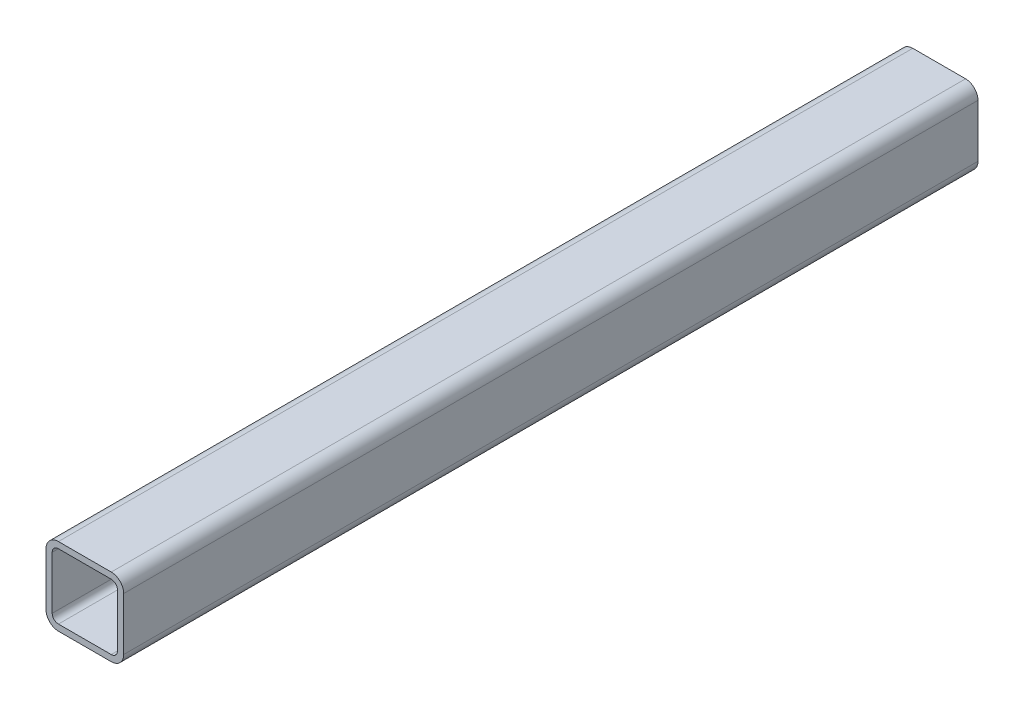
from build123d import *

# Parameters (mm, degrees)
BOSS_EXTRUDE1_DEPTH = 275


with BuildPart() as part:
    # Sketch1 → Boss-Extrude1 (new, symmetric)
    with BuildSketch(Plane.XY):
        with BuildLine():
            Line((-17, -25), (17, -25))
            ThreePointArc((17, -25), (22.656854249, -22.656854249), (25, -17))
            Line((25, -17), (25, 17))
            ThreePointArc((25, 17), (22.656854249, 22.656854249), (17, 25))
            Line((17, 25), (-17, 25))
            ThreePointArc((-17, 25), (-22.656854249, 22.656854249), (-25, 17))
            Line((-25, 17), (-25, -17))
            ThreePointArc((-25, -17), (-22.656854249, -22.656854249), (-17, -25))
        make_face()
        with BuildLine():
            Line((-17, 21), (17, 21))
            ThreePointArc((17, 21), (19.828427125, 19.828427125), (21, 17))
            Line((21, 17), (21, -17))
            ThreePointArc((21, -17), (19.828427125, -19.828427125), (17, -21))
            Line((17, -21), (-17, -21))
            ThreePointArc((-17, -21), (-19.828427125, -19.828427125), (-21, -17))
            Line((-21, -17), (-21, 17))
            ThreePointArc((-21, 17), (-19.828427125, 19.828427125), (-17, 21))
        make_face(mode=Mode.SUBTRACT)
    extrude(amount=BOSS_EXTRUDE1_DEPTH, both=True)


solid = part.part
